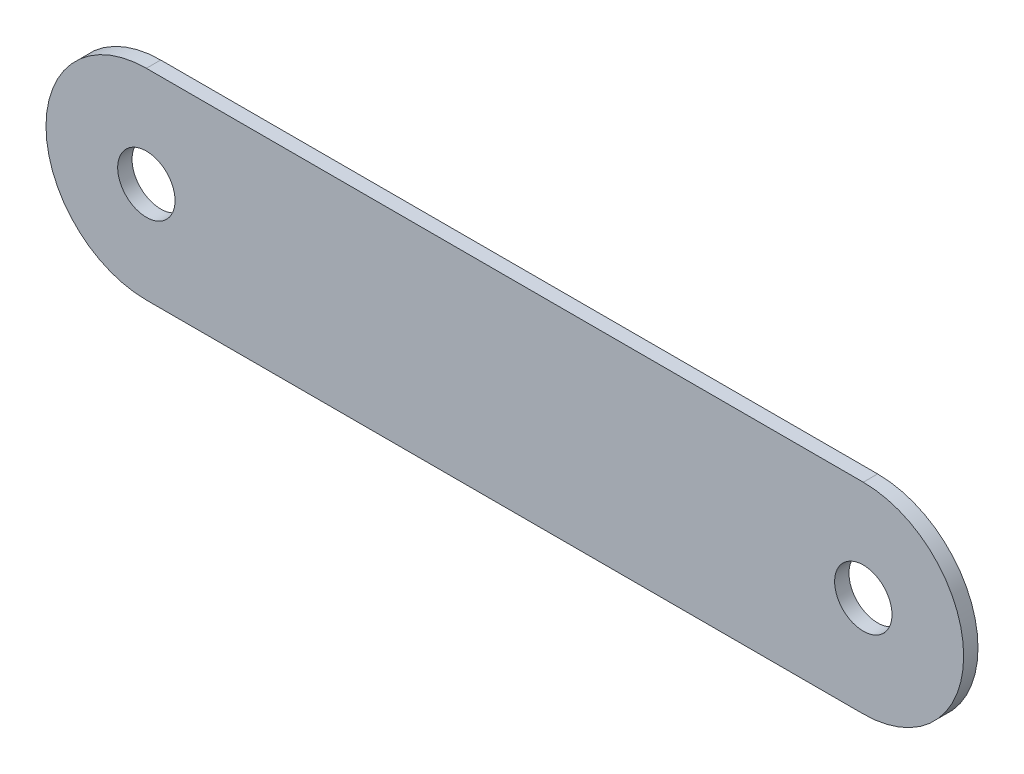
SolidWorks part; units mm, degrees
ref_plane "Front Plane" through (0, 0, 0) normal (0, 0, 1) x (1, 0, 0)
ref_plane "Top Plane" through (0, 0, 0) normal (0, 1, 0) x (1, 0, 0)
ref_plane "Right Plane" through (0, 0, 0) normal (1, 0, 0) x (0, 0, -1)
other "Configuration Table"
sketch "Sketch1" plane through (0, 0, 0) normal (0, 0, 1) x (1, 0, 0)
  line L0 (-33.1391, 0) -> (16.8609, 0) construction
  line L2 (-33.1391, 7) -> (16.8609, 7)
  line L3 (-33.1391, -7) -> (16.8609, -7)
  arc A0 (-33.1391, 7) -> (-33.1391, -7) centre (-33.1391, 0) ccw
  arc A1 (16.8609, -7) -> (16.8609, 7) centre (16.8609, 0) ccw
  circle A2 centre (-33.1391, 0) radius 2
  circle A3 centre (16.8609, 0) radius 2
  point P5 (-8.1391, 0)
extrude "Boss-Extrude1" add sketch "Sketch1" along normal blind 1
